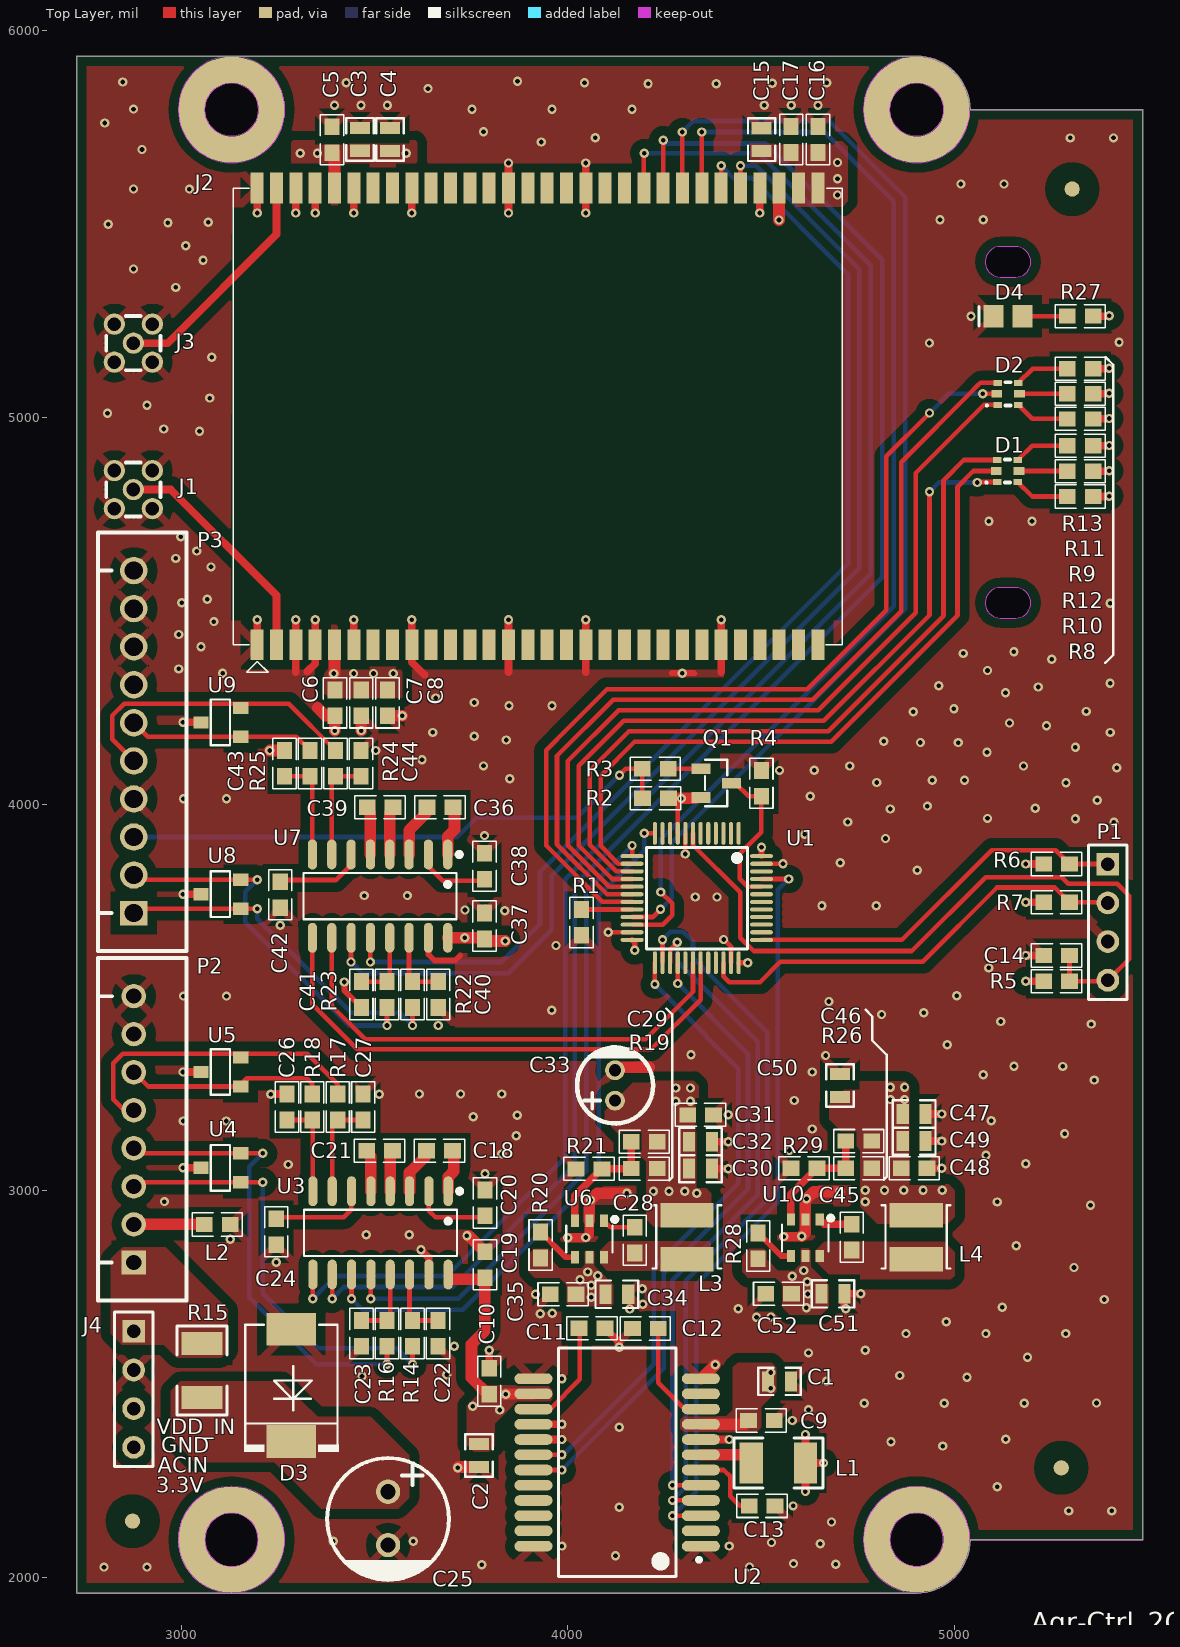
[diagram p0: Top Layer view]
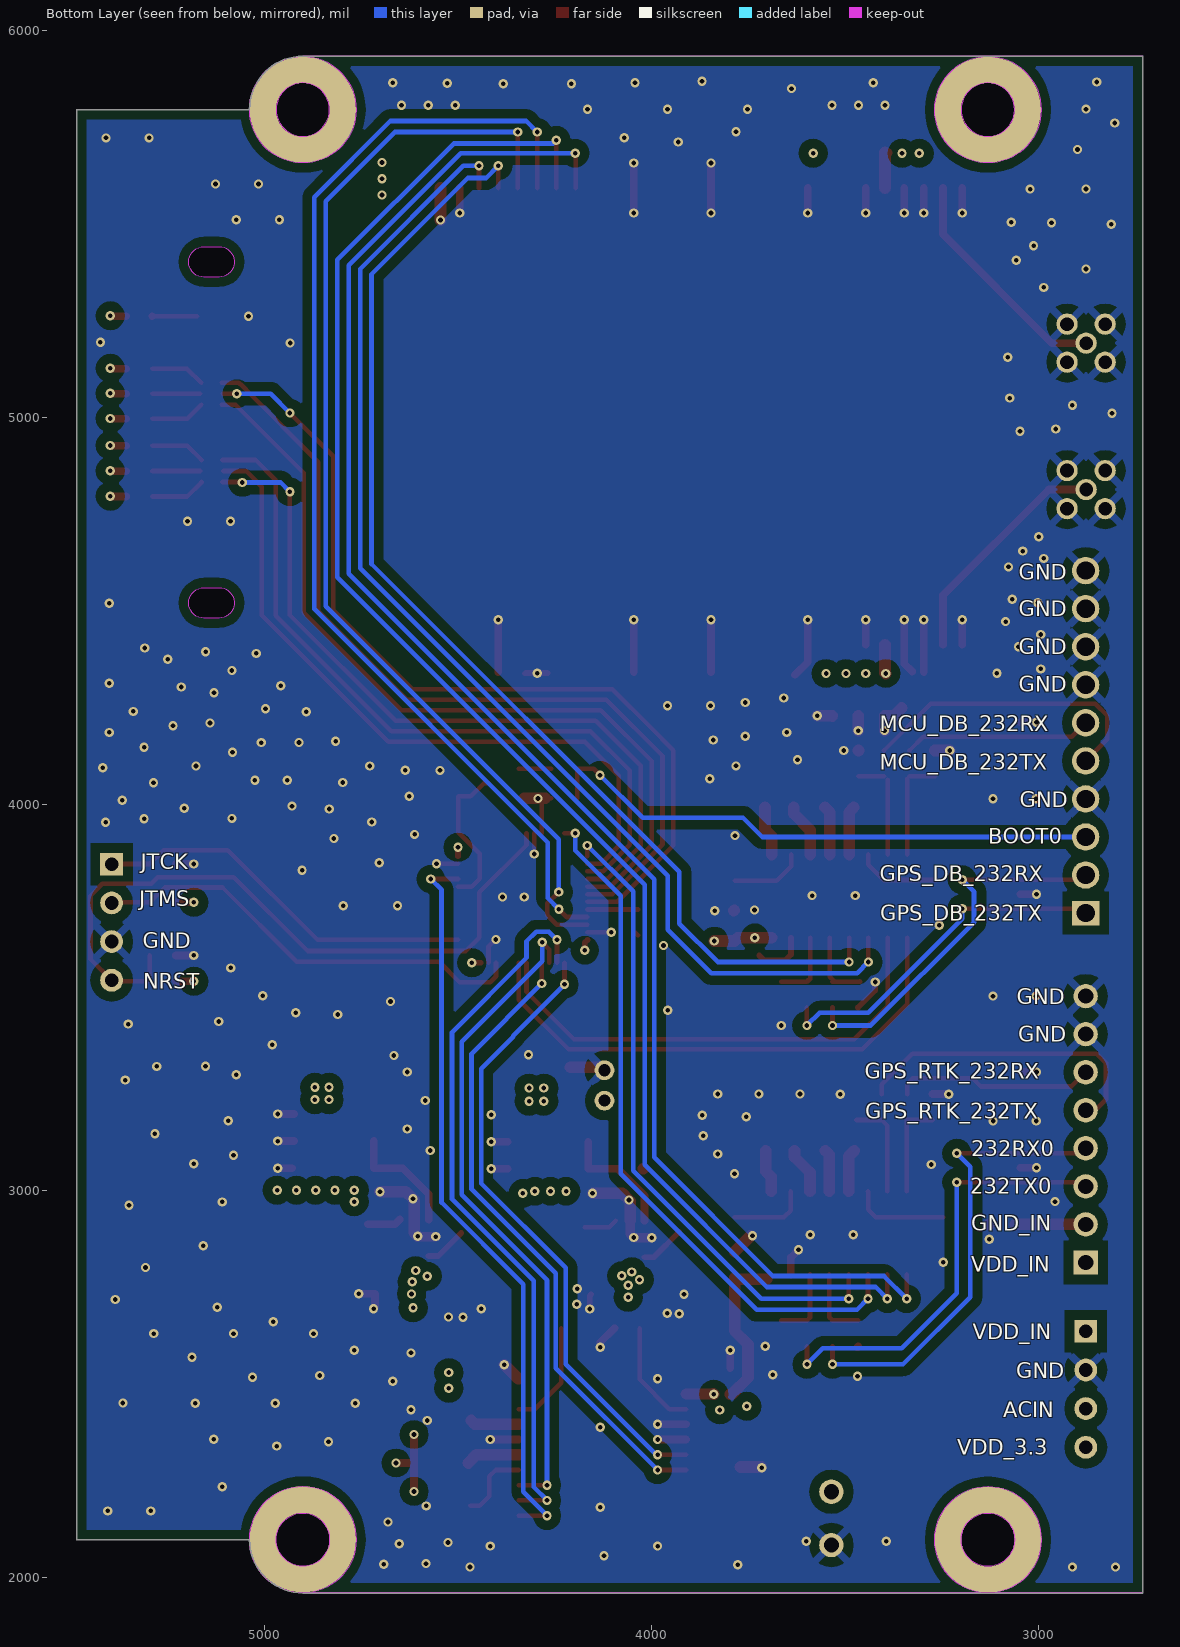
[diagram p1: Bottom Layer view, seen from below]
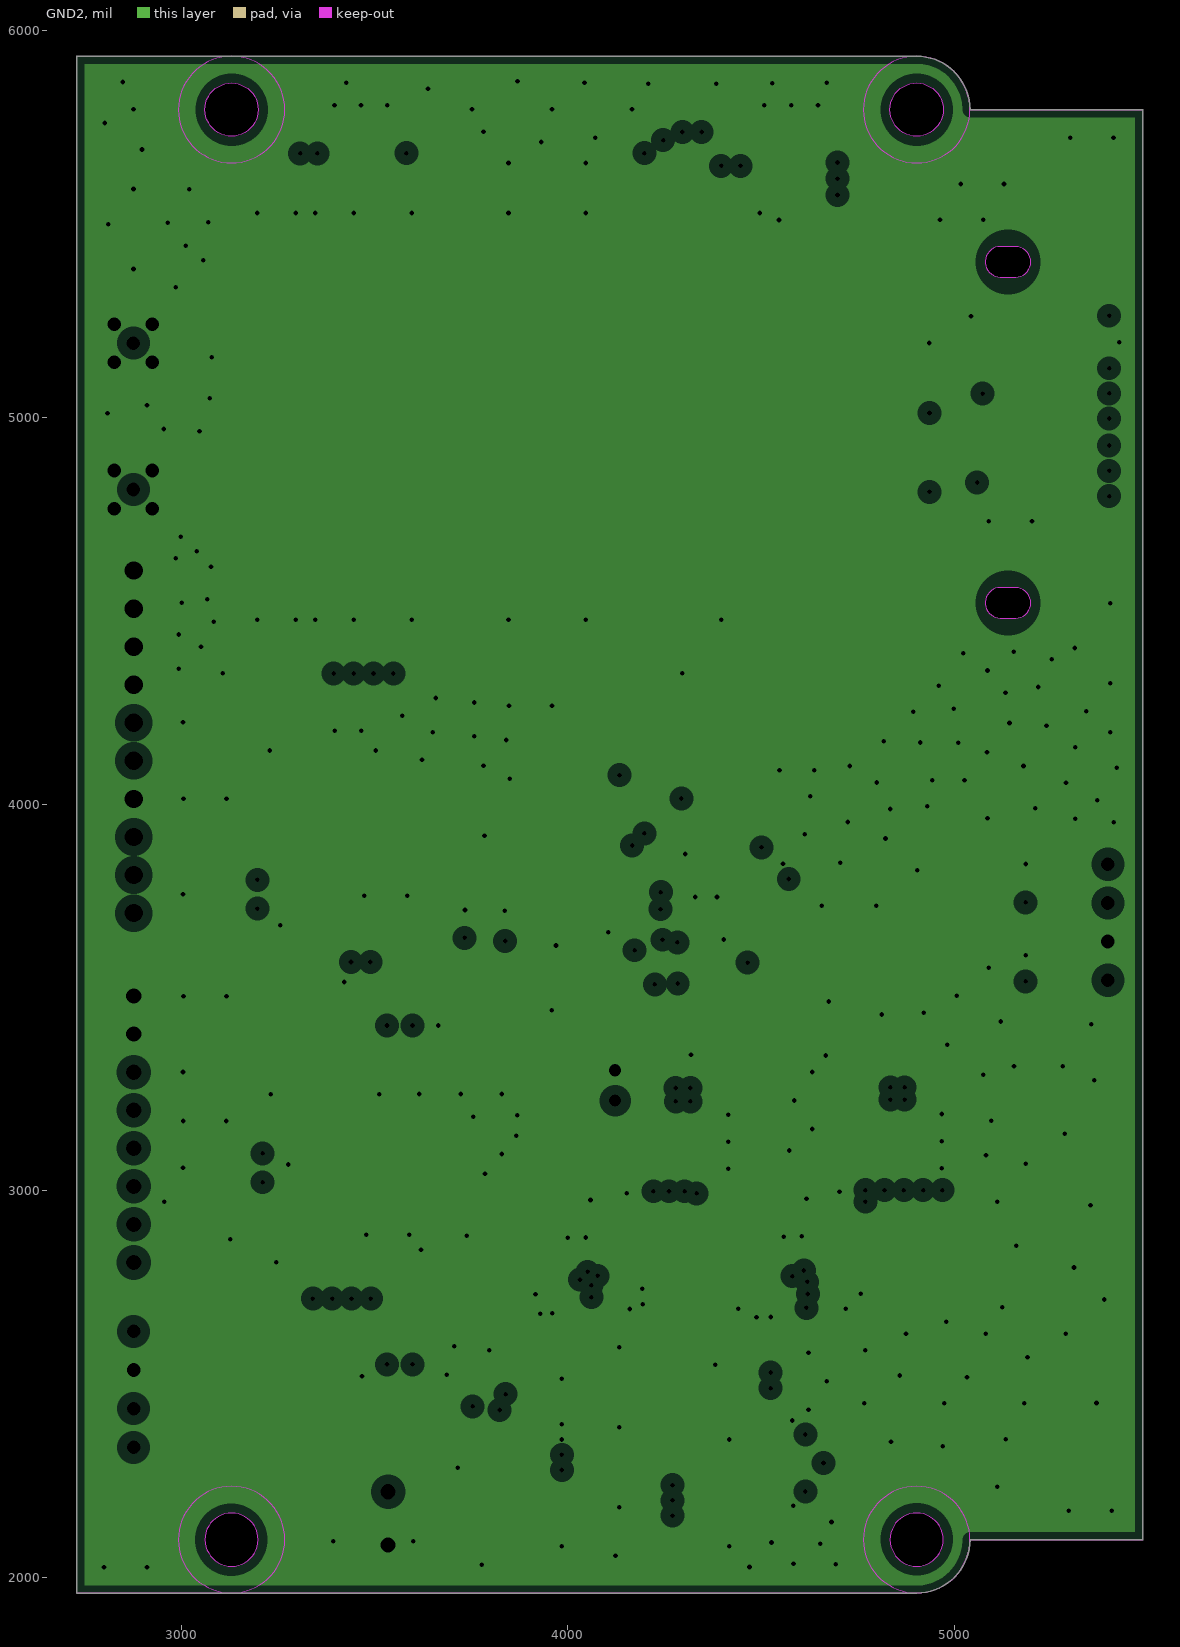
[diagram p2: GND2, clearances drawn from the general rule]
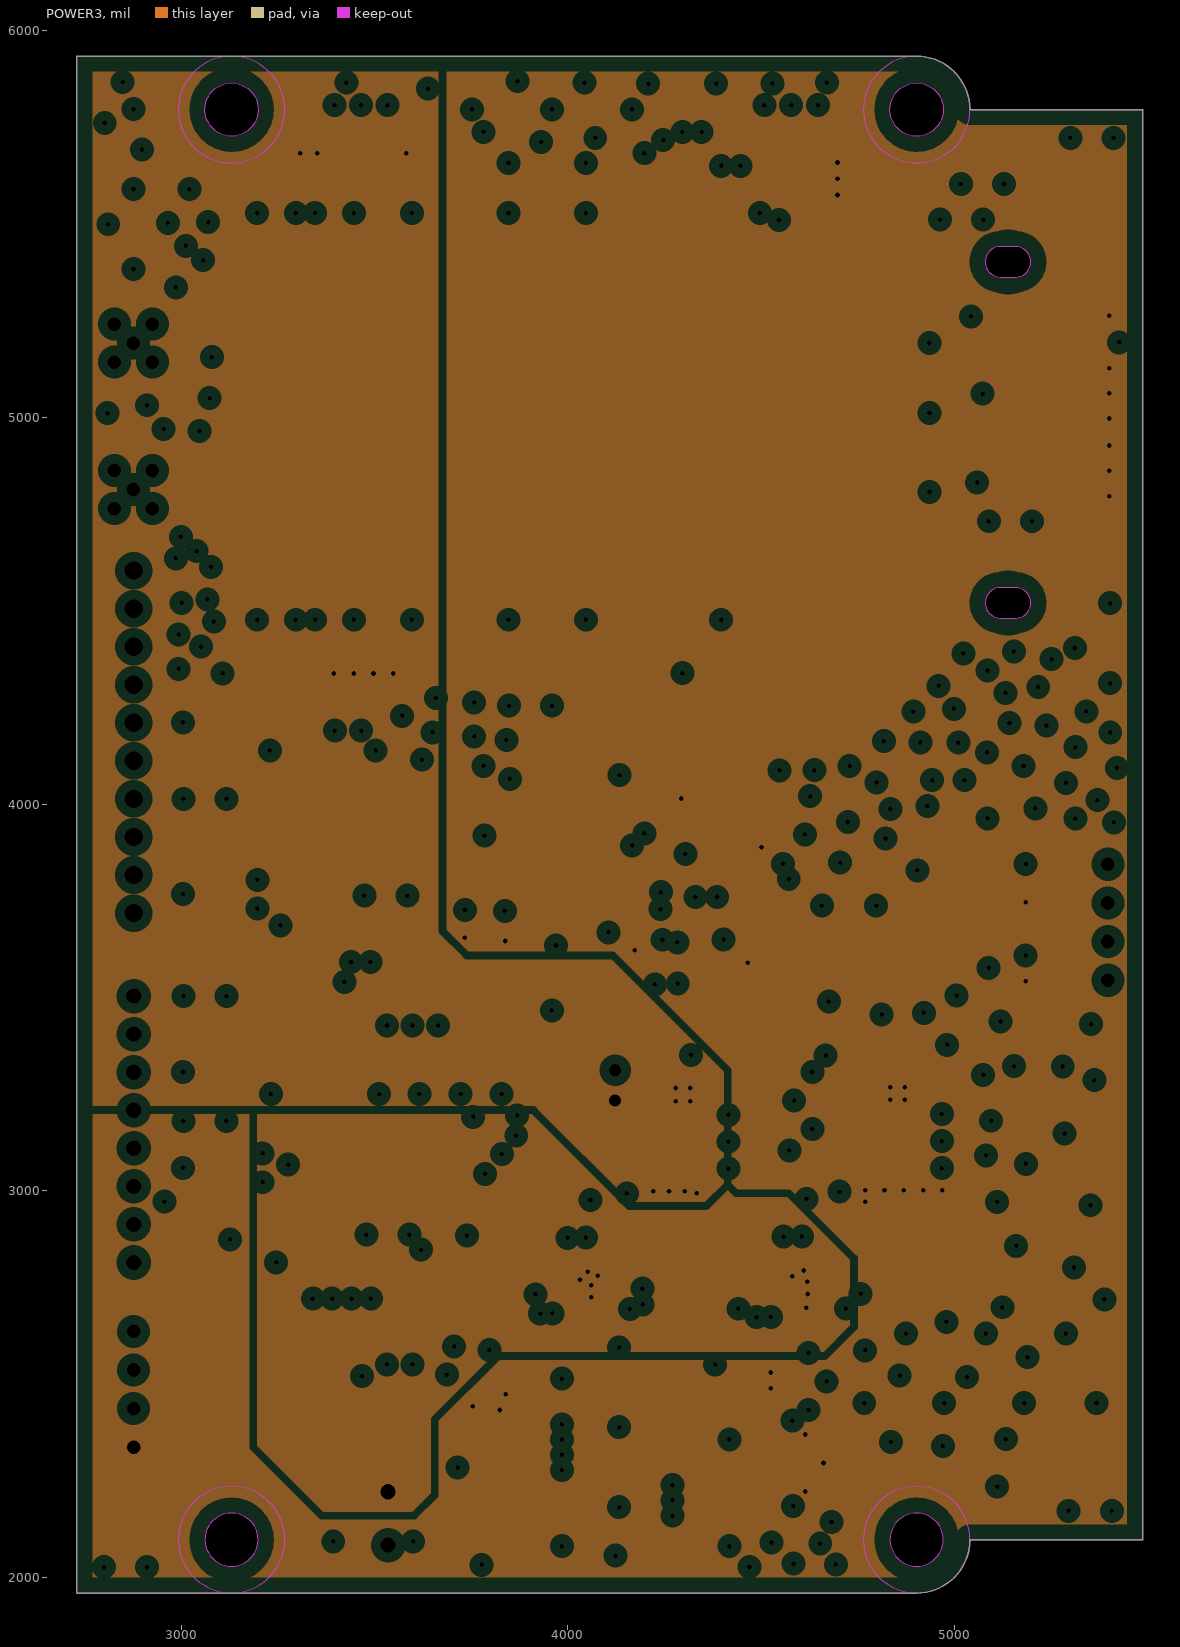
[diagram p3: POWER3, clearances drawn from the general rule]
# Altium PCB MISC84436.PcbDoc (part 1 of 2)
Units mil, origin at the board's own origin, x right, y up, seen from the top; angles counter-clockwise.
Board outline 2756.44 x 3974.35 mil, 4 copper layers (Top Layer, GND2, POWER3, Bottom Layer), stack 23.756 mil thick; 107 components, 89 nets, 422 pads, 390 vias.

## Layer stack, top to bottom
Top Layer: signal copper 1.4
Dielectric: prepreg 2.8, PP-006, Dk 4.1
GND2: plane copper 1.3778, net GND
Dielectric: dielectric 12.6, FR-4, Dk 4.8
POWER3: plane copper 1.3778, net (Multiple Nets)
Dielectric: prepreg 2.8, PP-006, Dk 4.1
Bottom Layer: signal copper 1.4

## Board outline
2730,1959.73 cw(c2730,1960) 2729.74,1960 2729.74,5933.82 cw(c2730,5933.82) 2730,5934.08 4901.63,5934.08 cw(c4901.63,5796.02) 5039.69,5796.29 5485.91,5796.29 cw(c5485.91,5796.02) 5486.17,5796.02 5486.17,2097.8 cw(c5485.91,2097.8) 5485.91,2097.53 5039.69,2097.53 cw(c4901.63,2097.8) 4901.63,1959.73 cw(c4901.63,2097.8) 4901.46,1959.73
cut-out: 3061.08,2097.8 ccw(c3129.97,2097.8) 3129.97,2028.9 ccw(c3129.97,2097.8) 3198.87,2097.8 ccw(c3129.97,2097.8) 3129.97,2166.69 ccw(c3129.97,2097.8)
cut-out: 4832.73,2097.8 ccw(c4901.63,2097.8) 4901.63,2028.9 ccw(c4901.63,2097.8) 4970.52,2097.8 ccw(c4901.63,2097.8) 4901.63,2166.69 ccw(c4901.63,2097.8)
cut-out: 4901.63,5727.12 cw(c4901.63,5796.02) 4832.73,5796.02 cw(c4901.63,5796.02) 4901.63,5864.92 cw(c4901.63,5796.02) 4970.52,5796.02 cw(c4901.63,5796.02)
cut-out: 3129.97,5727.12 cw(c3129.97,5796.02) 3061.08,5796.02 cw(c3129.97,5796.02) 3129.97,5864.92 cw(c3129.97,5796.02) 3198.87,5796.02 cw(c3129.97,5796.02)
cut-out: 5118.15,5362.95 5157.52,5362.95 ccw(c5157.52,5402.32) 5157.52,5441.69 5118.15,5441.69 ccw(c5118.15,5402.32)
cut-out: 5118.15,4481.06 5157.52,4481.06 ccw(c5157.52,4520.43) 5157.52,4559.8 5118.15,4559.8 ccw(c5118.15,4520.43)

## Design rules (kind name [scope] priority, off if disabled: settings)
Clearance mark [HASPAD('FREE-MARK')] p1: gap=50
Clearance GND_Clearance [InNet('GND')] p2: gap=6
Clearance [All] p3: gap=6
ComponentClearance [All] p1: gap=0 collisioncheckmode=3 verticalgap=0 showdistances=FALSE
HoleSize [All] p1: absolutevalues=TRUE maxlimit=500 minlimit=12 maxpercent=80.000 minpercent=20.000
HoleToHoleClearance [All] p1: gap=0 allowstackedmicrovias=TRUE
MinimumSolderMaskSliver [All] p1: minsoldermaskwidth=0
PlaneClearance [All] p1: clearance=25
PlaneConnect [All] p1: planeconnectstyle=Direct reliefexpansion=15 reliefentries=4 reliefconductorwidth=15 reliefairgap=15
PolygonConnect PolygonConnect_1 [ISVIA] p1: connectstyle=Direct reliefconductorwidth=10 reliefentries=4 polygonreliefangle="90 Angle"
PolygonConnect PolygonGND [InNet('GND')] p2: connectstyle=Relief reliefconductorwidth=20 reliefentries=4 polygonreliefangle="45 Angle"
PolygonConnect [All] p3: connectstyle=Direct reliefconductorwidth=10 reliefentries=4 polygonreliefangle="90 Angle"
RoutingVias [All] p1: holewidth=12 width=24 viastyle="Through Hole" minholewidth=12 minwidth=24 maxholewidth=12 maxwidth=24
SilkToSilkClearance [All] p1: silktosilkclearance=0
SilkscreenOverComponentPads SilkToSolderMaskClearance [IsPad] p1: minsilkscreentomaskgap=0
SolderMaskExpansion [All] p1: expansion=2.5
Width [All] p1: maxlimit=30 minlimit=6 preferedwidth=10
20 further rules are at their usual default settings.

## Components (designator, comment, footprint, x,y, rotation, side; value= is the part's Value field where it differs from the comment)
C1 "22uF/10V" C0805 4546.85,2507.09 r0 top
C2 "22uF/10V" C0805 3770.08,2315.3 r270 top
C3 "10uF/25V" C0805 3462.2,5719.29 r270 top
C4 "10uF/25V" C0805 3539.76,5718.9 r270 top
C5 "100nF/50V" 0603 3389.76,5718.11 r90 top
C6 "100pF/50V" 0603 3397.24,4261.81 r270 top
C7 "100pF/50V" 0603 3465.18,4261.81 r90 top
C8 "100nF/50V" 0603 3533.12,4261.81 r90 top
C9 "1uF/25V" 0603 4500,2405.91 r0 top
C10 "100nF/50V" 0603 3796.46,2507.48 r90 top
C11 "1uF/25V" 0603 4062.2,2644.49 r0 top
C12 "1uF/25V" 0603 4200,2643.7 r180 top
C13 "470nF/50V" 0603 4501.97,2185.04 r0 top
C14 "100nF/50V" 0603 5263.63,3608.66 r0 top
C15 "10uF/25V" C0805 4500.79,5718.5 r270 top
C16 "100pF/50V" 0603 4646.46,5718.9 r270 top
C17 "100nF/50V" 0603 4577.05,5718.9 r270 top
C18 "100nF/50V" 0603 3667.56,3103.66 r0 top
C19 "100nF/50V" 0603 3785.16,2808.56 r90 top
C20 "100nF/50V" 0603 3785.16,2968.56 r90 top
C21 "100nF/50V" 0603 3512.76,3103.66 r0 top
C22 "15pF/50V" 0603 3663.78,2631.14 r90 top
C23 "15pF/50V" 0603 3465.75,2631.14 r90 top
C24 "100nF/50V" 0603 3245.32,2894.13 r270 top
C25 "470uF/25V" CAP-TH_BD8.0-P3.50-D1.0-FD 3534.65,2152.76 r270 top
C26 "15pF/50V" 0603 3273.23,3216.54 r90 top
C27 "15pF/50V" 0603 3470.08,3216.54 r90 top
C28 "100nF/50V" 0603 4172.83,2872.28 r90 top
C29 "100pF/50V" 0603 4197.17,3126.8 r180 top
C30 "22uF/10V" C0805 4342.83,3057.28 r0 top
C31 "100nF/50V" 0603 4342.83,3196.31 r0 top
C32 "22uF/10V" C0805 4342.83,3126.8 r0 top
C33 "100uF/10V" CAP-TH_BD5.0-P2.00-D0.8-FD 4121.65,3272.44 r90 top
C34 "10uF/25V" C0805 4126.3,2732.28 r180 top
C35 "100nF/50V" 0603 3987.4,2732.28 r0 top
C36 "100nF/50V" 0603 3668.98,3991.83 r0 top
C37 "100nF/50V" 0603 3783.98,3684.63 r90 top
C38 "100nF/50V" 0603 3783.98,3839.43 r90 top
C39 "100nF/50V" 0603 3513.98,3991.83 r0 top
C40 "15pF/50V" 0603 3664.17,3507.48 r90 top
C41 "15pF/50V" 0603 3465.73,3507.48 r90 top
C42 "100nF/50V" 0603 3255.91,3765.75 r270 top
C43 "15pF/50V" 0603 3266.93,4105.24 r90 top
C44 "15pF/50V" 0603 3464.57,4105.24 r90 top
C45 "100nF/50V" 0603 4733.7,2880 r90 top
C46 "100pF/50V" 0603 4751.97,3128.46 r180 top
C47 "22uF/10V" C0805 4895.24,3198.46 r0 top
C48 "100nF/50V" 0603 4895.24,3058.46 r0 top
C49 "22uF/10V" C0805 4895.24,3128.46 r0 top
C50 "22uF/10V" C0805 4703.54,3272.44 r90 top
C51 "10uF/25V" C0805 4685.2,2733.46 r180 top
C52 "100nF/50V" 0603 4544.76,2733.46 r0 top
D1 "Full-color RGB LED" RGB 5137.01,4861.42 r180 top
D2 "Full-color RGB LED" RGB 5138.19,5061.02 r180 top
D3 "SMCJ18A" SMC_L6.9-W5.9-LS7.9-RD 3284.65,2496.85 r90 top
D4 "RED" LED_0805 5137.8,5261.81 r180 top
J1 "MMCX-KE RF connector" MMCX-TH_ZC11.801KK 2875.98,4813.39 r180 top
J2 "UM482/K823" UM482/K823 3921.06,5002.76 r90 top locked
J3 "MMCX-KE RF connector" MMCX-TH_ZC11.801KK 2875.98,5192.13 r0 top
J4 "Header" HDR1X4 2876.77,2636.61 r270 top
L1 "47uH±20%" 1210 4544.02,2296.06 r180 top
L2 "120Ω ±25% @100MHz" 0603 3092.91,2912.6 r0 top
L3 "2.2uH/2A" IND-SMD_L4.0-W4.0 4307.48,2879.92 r90 top
L4 "2.2uH/2A" IND-SMD_L4.0-W4.0 4900.39,2879.92 r90 top
P1 "Header" HDR1X4 5396.06,3844.49 r270 top locked
P2 "XH-8A" CONN-TH_XH-8A 2877.16,3159.06 r90 top locked
P3 "XH-10A" CONN-TH_10P-P2.50_XH-10A 2877.17,4161.03 r90 top locked
Q1 "8550" SOT-23-SS8550 4383.07,4054.33 r180 top
R1 "10K" 0603 4035.04,3694.09 r90 top
R2 "10K" 0603 4226.14,4015.12 r0 top
R3 "10K" 0603 4225.75,4091.5 r180 top
R4 "10K" 0603 4500.16,4053.7 r270 top
R5 "10K" 0603 5263.63,3541.73 r180 top
R6 "10K" 0603 5263.63,3845.28 r180 top
R7 "10K" 0603 5263.63,3746.06 r180 top
R8 "1.5K" 0603 5324.8,4795.47 r180 top
R9 "1.5K" 0603 5324.8,4996.26 r180 top
R10 "680R" 0603 5324.8,4861.02 r180 top
R11 "680R" 0603 5324.8,5061.22 r180 top
R12 "1K" 0603 5324.8,4926.57 r180 top
R13 "1K" 0603 5324.8,5126.18 r180 top
R14 "4.7Ω,±1%" 0603 3597.77,2631.14 r90 top
R15 "12V/2A" 1210 3053.54,2535.43 r90 top
R16 "4.7Ω,±1%" 0603 3531.76,2631.14 r90 top
R17 "4.7Ω,±1%" 0603 3404.46,3216.54 r270 top
R18 "4.7Ω,±1%" 0603 3338.85,3216.54 r270 top
R19 "75K 1%" 0603 4197.17,3057.28 r0 top
R20 "100K" 0603 3929.13,2859.84 r270 top
R21 "10K" 0603 4054.25,3056.65 r0 top
R22 "4.7Ω,±1%" 0603 3598.02,3507.48 r90 top
R23 "4.7Ω,±1%" 0603 3531.88,3507.48 r90 top
R24 "4.7Ω,±1%" 0603 3398.69,4105.24 r270 top
R25 "4.7Ω,±1%" 0603 3332.81,4105.24 r270 top
R26 "100K" 0603 4751.97,3058.46 r0 top
R27 "1K" 0603 5324.8,5262.01 r0 top
R28 "100K" 0603 4491.73,2857.48 r270 top
R29 "22.1K" 0603 4610.24,3058.46 r0 top
U1 "STM32F103C8T6/GD32F103C8T6" LQFP-48_L7.0-W7.0-P0.50-LS9.0-BL 4333.08,3757.09 r180 top locked
U2 "SCC2130" SCC2130D 4127.15,2297.63 r180 top
U3 "SP3232EEN" SOP16-6.6 3515.16,2891.16 r270 top
U4 "PESD15VL2BT" SOT-23 3102.24,3059.45 r90 top
U5 "PESD15VL2BT" SOT-23 3102.24,3307.09 r90 top
U6 "SY8113B" TSOT-23-6_L2.9-W1.6-P0.95-LS2.8-BR 4055.19,2875.32 r90 top
U7 "SP3232EEN" SOP16-6.6 3513.98,3762.03 r270 top
U8 "PESD15VL2BT" SOT-23 3102.24,3766.93 r90 top
U9 "PESD15VL2BT" SOT-23 3102.24,4211.42 r90 top
U10 "SY8113B" TSOT-23-6_L2.9-W1.6-P0.95-LS2.8-BR 4613.7,2878.46 r90 top

## Footprints (in the part's own frame and the unit in brackets; to place one, negate y for a bottom-side part, rotate by r counter-clockwise, add the part's x,y. Pads: shape width x height; smd on the part's side, far side on the other; paste and mask are expansions set on the pad)
0603 [mm] "贴片带丝印"
  rect 1.1x1 smd: 1(-0.85,0) 2(0.85,0)
  silkscreen extent -1.65,-0.76 1.65,0.76, body extent -1.14,-0.38 1.14,0.38, height 1
1210 [mil] "贴片元件"
  rect 60x106.3 smd: 1(-70,0) 2(70,0)
  silkscreen extent -115,-65 115,65, body extent -65,-50 65,50, height 39
C0805 [mm] "C0805"
  rect 0.8x1.3 smd: 1(-0.75,0) 2(0.75,0)
  silkscreen extent -1.4,-0.9 1.4,0.9
CAP-TH_BD5.0-P2.00-D0.8-FD [mm]
  round 1.3 hole 0.8: 1(-1,0) 2(1,0)
  silkscreen extent -2.5,-2.5 2.5,2.5
CAP-TH_BD8.0-P3.50-D1.0-FD [mm]
  round 1.6 hole 1: 1(-1.75,0) 2(1.75,0)
  silkscreen extent -3.96,-4 4.04,4
CONN-TH_10P-P2.50_XH-10A [mm]
  rect 1.6x1.8 hole 1.2: 1(-11.25,0)
  round 1.8 hole 1.2: 2(-8.75,0) 3(-6.25,0) 4(-3.75,0) 5(-1.25,0) 6(1.25,0) 7(3.75,0) 8(6.25,0) 9(8.75,0) 10(11.25,0)
  silkscreen extent -13.75,-3.45 13.75,2.35
CONN-TH_XH-8A [mm]
  rect 1.6x1.6 hole 1: 1(-8.75,0)
  round 1.6 hole 1: 2(-6.25,0) 3(-3.75,0) 4(-1.25,0) 5(1.25,0) 6(3.75,0) 7(6.25,0) 8(8.75,0)
  silkscreen extent -11.25,-3.46 11.25,2.35
HDR1X4 [mm] "Connector; Header; 4 Position"
  rect 1.5x1.5 hole 0.9: 1(0,0)
  round 1.5 hole 0.9: 2(2.54,0) 3(5.08,0) 4(7.62,0)
  silkscreen extent -1.27,-1.27 8.89,1.27
IND-SMD_L4.0-W4.0 [mm]
  rect 1.6x3.5 smd: 1(-1.45,0) 2(1.45,0)
  silkscreen extent -2.05,-2.25 2.1,2.25
LED_0805 [mm] "贴片二极管"
  rect 1.3x1.5 smd: 1(-0.95,0) 2(0.95,0)
  silkscreen extent 1.91,-0.63 1.91,0.64
LQFP-48_L7.0-W7.0-P0.50-LS9.0-BL [mm]
  oval 0.27x1.5 smd: 1(-2.75,-4.25) 2(-2.25,-4.25) 3(-1.75,-4.25) 4(-1.25,-4.25) 5(-0.75,-4.25) 6(-0.25,-4.25) 7(0.25,-4.25) 8(0.75,-4.25) 9(1.25,-4.25) 10(1.75,-4.25) 11(2.25,-4.25) 12(2.75,-4.25) 25(2.75,4.25) 26(2.25,4.25) 27(1.75,4.25) 28(1.25,4.25) 29(0.75,4.25) 30(0.25,4.25) 31(-0.25,4.25) 32(-0.75,4.25) 33(-1.25,4.25) 34(-1.75,4.25) 35(-2.25,4.25) 36(-2.75,4.25)
  oval 1.5x0.27 smd: 13(4.25,-2.75) 14(4.25,-2.25) 15(4.25,-1.75) 16(4.25,-1.25) 17(4.25,-0.75) 18(4.25,-0.25) 19(4.25,0.25) 20(4.25,0.75) 21(4.25,1.25) 22(4.25,1.75) 23(4.25,2.25) 24(4.25,2.75) 37(-4.25,2.75) 38(-4.25,2.25) 39(-4.25,1.75) 40(-4.25,1.25) 41(-4.25,0.75) 42(-4.25,0.25) 43(-4.25,-0.25) 44(-4.25,-0.75) 45(-4.25,-1.25) 46(-4.25,-1.75) 47(-4.25,-2.25) 48(-4.25,-2.75)
  silkscreen extent -3.33,-3.31 3.3,3.34
MMCX-TH_ZC11.801KK [mm]
  round 1.4 hole 0.9: 1(0,0) 2(-1.25,1.25) 3(1.25,1.25) 4(1.25,-1.25) 5(-1.25,-1.25)
  silkscreen extent -1.78,-1.78 1.78,1.78
RGB [mm]
  rect 0.55x0.4 smd: 1(0.675,0.725) 2(-0.675,0.725) 5(0.675,-0.725) 6(-0.675,-0.725)
  rect 0.7x0.5 smd: 3(0.75,0) 4(-0.75,0)
  silkscreen extent -0.17,-0.76 1.46,0.82
SCC2130D [mm] "SOP, 24-Leads, Body 15.00x8.50mm, Pitch 1.00mm, IPC Medium Density"
  oval 2.5x0.7 smd: 1(-5.5,5.5) 2(-5.5,4.5) 3(-5.5,3.5) 4(-5.5,2.5) 5(-5.5,1.5) 6(-5.5,0.5) 7(-5.5,-0.5) 8(-5.5,-1.5) 9(-5.5,-2.5) 10(-5.5,-3.5) 11(-5.5,-4.5) 12(-5.5,-5.5) 13(5.5,-5.5) 14(5.5,-4.5) 15(5.5,-3.5) 16(5.5,-2.5) 17(5.5,-1.5) 18(5.5,-0.5) 19(5.5,0.5) 20(5.5,1.5) 21(5.5,2.5) 22(5.5,3.5) 23(5.5,4.5) 24(5.5,5.5)
  silkscreen extent -5.5,-7.5 3.85,7.5, body extent -4.25,-7.5 4.25,7.5, height 4.2
SMC_L6.9-W5.9-LS7.9-RD [mm]
  rect 2.158x3.24 smd: 1(3.686,0) 2(-3.686,0)
  silkscreen extent -4.36,-3.1 3.98,3.1
SOP16-6.6 [mil]
  oval 77.6x23.7 smd: 1(-107.7,175) 2(-107.7,125) 3(-107.7,75) 4(-107.7,25) 5(-107.7,-25) 6(-107.7,-75) 7(-107.7,-125) 8(-107.7,-175) 9(107.7,-175) 10(107.7,-125) 11(107.7,-75) 12(107.7,-25) 13(107.7,25) 14(107.7,75) 15(107.7,125) 16(107.7,175)
  silkscreen extent -114,-198 60,211
SOT-23 [mm] "SOT-23"
  rect 0.8x1 smd: 1(-0.95,-1.3) 2(0.95,-1.3) 3(0,1.3)
  silkscreen extent -1.5,-0.61 1.5,0.66
SOT-23-SS8550 [mm]
  rect 1.25x0.7 smd: 1(1,-0.95) 2(1,0.95) 3(-1,0)
  silkscreen extent -0.73,-1.53 0.73,1.53
TSOT-23-6_L2.9-W1.6-P0.95-LS2.8-BR [mm]
  rect 0.8x0.532 smd: 1(1.2,-0.95) 2(1.2,0) 3(1.2,0.95) 4(-1.2,0.95) 5(-1.2,0) 6(-1.2,-0.95)
  silkscreen extent -0.88,-1.82 1.44,1.53
UM482/K823 [mm]
  rect 2.01x0.85 smd: 1(-15,18.415) 2(-15,17.145) 3(-15,15.875) 4(-15,14.605) 5(-15,13.335) 6(-15,12.065) 7(-15,10.795) 8(-15,9.525) 9(-15,8.255) 10(-15,6.985) 11(-15,5.715) 12(-15,4.445) 13(-15,3.175) 14(-15,1.905) 15(-15,0.635) 16(-15,-0.635) 17(-15,-1.905) 18(-15,-3.175) 19(-15,-4.445) 20(-15,-5.715) 21(-15,-6.985) 22(-15,-8.255) 23(-15,-9.525) 24(-15,-10.795) 25(-15,-12.065) 26(-15,-13.335) 27(-15,-14.605) 28(-15,-15.875) 29(-15,-17.145) 30(-15,-18.415) 31(15,-18.415) 32(15,-17.145) 33(15,-15.875) 34(15,-14.605) 35(15,-13.335) 36(15,-12.065) 37(15,-10.795) 38(15,-9.525) 39(15,-8.255) 40(15,-6.985) 41(15,-5.715) 42(15,-4.445) 43(15,-3.175) 44(15,-1.905) 45(15,-0.635) 46(15,0.635) 47(15,1.905) 48(15,3.175) 49(15,4.445) 50(15,5.715) 51(15,6.985) 52(15,8.255) 53(15,9.525) 54(15,10.795) 55(15,12.065) 56(15,13.335) 57(15,14.605) 58(15,15.875) 59(15,17.145) 60(15,18.415)
  silkscreen extent -16.81,-20 15,20

## Part data
C1 C2 C30 C32: library part Cap, "SMD ceramic capacitor,X5R"
C3 C4 C9 C10 C11 C12 C13 C15: library part Cap, "SMD ceramic capacitor,X7R"
C5 C6 C7 C8 C16 C17 C28 C29 C31 C35: library part Cap, "SMD ceramic capacitor"
C14 C45 C46 C47 C48 C49 C51 C52: library part Cap, "Capacitor"
C18 C19 C20 C21 C22 C23 C24 C26 C27 C36 C37 C38 C39 C40 C41 C42 C43 C44: library part Cap, "SMD capacitor,X7R"
C25: library part Cap, "470μF,25V,Ф8×11.5mm,RoHS"
C33: library part Cap2, "100μF,10V,Ф5×7mm,RoHS"
C34: library part Cap, "SMD ceramic capacitor,MLCC"
C50: library part Cap2, "Capacitor"
D1 D2: library part LED1_3, "19-337C/RSBHGHC-M03/2T,EVERLIGHT (Taiwan)"
D3: library part Diode, "TVS diode"
D4: library part LED1, "Red high-brightness LED"
J1 J3: library part CIRCLE
J2: library part UM482, "High-precision GNSS receiver"
J4: library part 2.54, "Single-row straight header,4P,2.54mm"
L1: library part Inductor, "SMD inductor"
L2: library part Inductor, "Ferrite bead"
L3 L4: library part Inductor, "SMD power inductor,cjiang,FNR4026S2R2MT"
P1: library part "Header 4", "Single-row straight header,4P,2.54mm"
P2: library part "Header 8", "8P,pitch 2.5mm,through-hole,BOOMELE"
P3: library part "Header 10", "10P,pitch 2.5mm,through-hole,BOOMELE"
Q1: library part PNP, "PNP Bipolar Transistor"
R1 R2 R3 R4 R5: library part Res, "SMD resistor"
R6 R7 R8 R9 R10 R11 R12 R13 R19 R20 R21 R26 R27 R28 R29: library part Res1, "SMD resistor"
R14 R16 R17 R18 R22 R23 R24 R25: library part RES, "SMD resistor"
R15: library part RES, "Resettable fuse"
U1: library part STM32F103C8T6, "STM32 ARM-based 32-bit MCU with ST/GD GigaDevice"
U2: "MEMS digital gyroscope"
U3 U7: library part SP202ECT
U4 U5 U8 U9: library part PESD12VL2BT

## Free pads (board coordinates)
  round 40 hole 78.74 slot 118.11 at 0 deg unplated: 0(5137.8,4520.47) 0(5137.8,5402.36)
  round 275.59 hole 137.8 unplated: 1(3129.53,2097.64) 1(3130.31,5795.67) 1(4901.57,2098.43) 1(4901.57,5796.06)
  round 39.37 smd mask+59.06: MARK(2874.02,2145.67) MARK(5275.59,2283.46) MARK(5303.94,5590.55)

## Via types
v1: diameter 24, hole 12, Top Layer to Bottom Layer, tented both sides, 252 vias
v2: diameter 24, hole 12, Top Layer to Bottom Layer, 138 vias

## Nets (pads, with @x,y where several pads share a name; then routed paths per layer and width w, separated by ;. In a path a pad name is that pad's centre, name@x,y a point inside that pad or via, vN(x,y) a via of type N, cw(c..) or ccw(c..) an arc to the next point about the centre after c; other vN are vias at no path point)
232RX0: P2.4 R16.1 U4.2 | length 1199.2
  Top Layer w12: P2.4@2877.17,3109.84 2885.04,3109.84 2898.03,3096.85 U4.2@3153.43,3096.85 v1(3210.24,3096.85) ; v1(3531.76,2551.21) R16.1@3531.76,2597.68
  Bottom Layer w12: v1(3210.24,3096.85) 3175.59,3062.2 3175.59,2725.2 3349.57,2551.21 v1(3531.76,2551.21)
232TX0: P2.3 R14.1 U4.1 | length 1135
  Top Layer w12: P2.3@2877.17,3011.42 2887.8,3022.05 U4.1@3153.43,3022.05 v1(3210.24,3022.05) ; v1(3597.91,2551.21) R14.1@3597.91,2597.68
  Bottom Layer w12: v1(3210.24,3022.05) 3210.24,2734.64 3352.36,2592.52 3556.6,2592.52 v1(3597.91,2551.21)
ACIN: J4.3
BOOT0: P3.3 R2.1 R3.2 | length 1464.8
  Top Layer w12: v1(4133.07,4074.8) 4149.76,4091.5 R3.2@4192.28,4091.5 4192.28,4015.51 R2.1@4192.68,4015.12
  Bottom Layer w12: P3.3@2877.17,3914.96 3713.78,3914.96 3763.39,3964.57 4022.83,3964.57 v1(4133.07,4074.8)
CPU-URX0: U1.31 U7.9 | length 1372.8
  Top Layer w12: U7.9@3338.98,3654.33 3338.98,3481.89 3454.72,3366.14 4214.57,3366.14 4342.91,3494.49 U1.31@4342.91,3589.78
CPU-UTX0: U1.30 U7.10 | length 1272.4
  Top Layer w12: U7.10@3388.98,3654.33 3388.98,3477.95 3475.2,3391.73 4200.39,3391.73 4323.24,3514.58 U1.30@4323.24,3589.78
GND: C1.2 C2.2 C3.1 C4.1 C5.2 C6.2 C7.1 C8.1 C9.2 C10.2 C11.2 C12.2 C13.2 C14.1 C15.1 C16.1 C17.1 C19.2 C20.2 C22.1 C23.1 C24.2 C25.2 C26.2 C27.2 C30.2 C31.2 C32.2 C33.2 C34.1 C35.1 C37.2 C38.2 C40.1 C41.1 C42.2 C43.2 C44.2 C47.2 C48.2 C49.2 C50.2 C51.1 C52.1 D3.1 D4.2 J1.2 J1.3 J1.4 J1.5 J2.1 J2.3 J2.4 J2.6 J2.9 J2.14 J2.18 J2.25 J2.33 J2.34 J2.43 J2.47 J2.52 J2.55 J2.57 J2.58 J2.60 J3.2 J3.3 J3.4 J3.5 J4.2 L2.2 P1.3 P2.7 P2.8 P3.4 P3.7 P3.8 P3.9 P3.10 R1.1 R4.1 R6.2 R21.1 R29.1 U1.8 U1.23 U1.35 U1.47 U2.1 U2.8 U2.12 U2.13 U2.16 U2.17 U2.24 U3.15 U4.3 U5.3 U6.2 U7.15 U8.3 U9.3 U10.2 | length 4279
  Top Layer w12: R1.1@4035.04,3660.63 R1.1@4042.92,3668.52 ; v1(4104.34,3668.52) U1.23@4165.75,3668.52 ; v1(4295.67,4338.58) 4296.85,4337.4 v1@4297.64,4337.4 ; v1@4296.06,4338.98 v1@4297.64,4337.4 ; v1(4303.54,3870.87) U1.8@4303.54,3924.41 ; 4328.35,4337.4 v1@4297.64,4337.4 ; v1(4402.36,3650) 4421.65,3630.71 U1.35@4421.65,3589.78 ; U1.47@4500.4,3845.67 v1@4555.51,3845.67 ; v1(5042.13,5261.42) v1@5042.52,5261.81
  Top Layer w15: v1(3421.65,3539.76) 3421.65,3518.09 C41.1@3465.73,3474.02 ; U7.15@3638.98,3654.33 3638.98,3611.02 3654.72,3595.28 3707.64,3595.28 3721.17,3608.8 ; C34.1@4155.83,2732.28 4159.76,2728.35 v1(4159.76,2694.09) ; 4325.98,4338.19 4325.2,4338.98 v1@4296.06,4338.98 ; v1@4552.76,2881.49 v1(4557.72,2881.49) ; v1@4296.06,4338.98 4268.9,4338.98 4268.5,4338.58 v1(4295.67,4338.58) v1@4296.06,4338.98
  Top Layer w20: v1(3004.33,3059.45) U4.3@3046.06,3059.45 ; v1(3004.33,3307.09) U5.3@3046.06,3307.09 ; v1(3004.33,3766.93) U8.3@3046.06,3766.93 ; v1(3004.33,4211.42) U9.3@3046.06,4211.42 ; J2.1@3196.06,4412.2 v1(3196.06,4476.77) ; v1(3196.06,5528.74) J2.60@3196.06,5593.31 ; v1(3231.5,3250) C26.2@3273.23,3250 ; 3296.06,4341.73 J2.3@3296.06,4412.2 v1(3296.06,4476.77) ; v1(3296.06,5528.74) J2.58@3296.06,5593.31 ; 3325.59,4342.91 3346.06,4363.39 J2.4@3346.06,4412.2 v1(3346.06,4476.77) ; v1(3346.06,5528.74) J2.57@3346.06,5593.31 ; J2.6@3446.06,4412.2 v1(3446.06,4476.77) ; v1(3446.06,5528.74) J2.55@3446.06,5593.31 ; C23.1@3464.96,2597.68 C23.1@3467.32,2595.32 ; v1(3596.06,4476.77) J2.9@3596.06,4412.2 3596.06,4367.32 3628.74,4334.65 ; v1(3596.06,5528.74) J2.52@3596.06,5593.31 ; v1(3619.68,2847.64) 3640.16,2827.17 U3.15@3640.16,2783.46 ; C10.2@3796.46,2540.94 v1(3796.46,2587.64) ; 3846.06,4341.73 J2.14@3846.06,4412.2 v1(3846.06,4476.77) ; v1(3846.06,5528.74) J2.47@3846.06,5593.31 v1(3846.06,5657.87) ; U2.17@3910.61,2356.69 v1(3984.21,2356.69) ; U2.16@3910.61,2396.06 v1(3984.21,2396.06) ; 4046.06,4341.73 J2.18@4046.06,4412.2 v1(4046.06,4476.77) ; v1(4046.06,5528.74) J2.43@4046.06,5593.31 v1(4046.06,5657.87) ; C11.2@4095.67,2644.49 4132.28,2607.87 ; U2.8@4343.69,2356.69 v1(4417.28,2356.69) ; C30.2@4372.36,3057.28 v1(4414.49,3057.28) ; C32.2@4372.36,3126.8 v1(4414.49,3126.8) ; 4396.06,4341.73 J2.25@4396.06,4412.2 v1(4396.06,4476.77) ; v1(4496.06,5528.74) J2.34@4496.06,5593.31 ; v1(4718.66,2695.28) 4714.72,2699.21 C51.1@4714.72,2733.46 v1(4756.85,2733.46) ; C49.2@4924.76,3128.46 v1(4966.89,3128.46) ; C47.2@4924.76,3198.46 v1(4966.89,3198.46) ; C48.2@4928.7,3058.46 v1(4966.89,3058.46) ; v1(5183.46,3608.66) C14.1@5230.16,3608.66 ; v1(5183.46,3845.28) R6.2@5230.16,3845.28
  Top Layer w25: v1(3999.21,2878.35) 4045.28,2878.35 v1(4046.06,2879.13) 4055.19,2888.26 U6.2@4055.19,2922.56 ; v1(4557.72,2881.49) 4603.79,2881.49 v1(4604.57,2882.28)
  Top Layer w30: L2.2@3125.98,2912.99 L2.2@3126.38,2912.6 ; v1(3228.74,4138.7) C43.2@3266.93,4138.7 C43.2@3267.32,4139.09 ; 3352.56,4248.62 3372.83,4228.35 C6.2@3397.24,4228.35 v1(3397.24,4190.16) ; C44.2@3464.17,4138.31 C44.2@3464.57,4138.7 ; C7.1@3464.79,4228.74 C7.1@3465.18,4228.35 v1(3465.18,4190.16) ; C8.1@3532.72,4227.95 C8.1@3533.12,4228.35 v1(3571.31,4228.35) ; v1@3716.49,2285.78 C2.2@3770.08,2285.78 ; v1@3743.33,2883.86 C19.2@3785.16,2842.03 ; C37.2@3785.83,3725.2 C37.2@3787.01,3724.02 ; R21.1@4020.79,3056.65 R21.1@4021.18,3057.05 ; U6.2@4055.19,2922.56 4055.19,2972.91 v1(4058.27,2975.98) 4075.59,2993.31 v1(4152.36,2993.31) ; C33.2@4121.65,3311.81 4129.53,3319.68 4210.24,3319.68 ; U2.12@4343.69,2514.17 4344.48,2514.17 v1(4380.71,2550.39) ; v1(4545.67,5510.63) 4545.67,5592.91 J2.33@4546.06,5593.31 ; v1(4604.57,2882.28) 4613.7,2891.41 U10.2@4613.7,2925.7 4613.7,2976.05 v1(4616.78,2979.13) 4635.29,2997.64 v1(4701.97,2997.64)
  other v1: 2800,2026.77 2911.42,2026.77 3776.77,2032.68 4122.83,2056.3 3984.21,2081.09 4417.28,2081.09 4526.38,2090.55 3392.91,2093.31 3599.68,2093.31 5294.88,2172.05 5406.3,2172.05 4132.28,2181.73 4582.13,2185.04 3714.57,2283.86 4132.28,2388.5 4580.16,2405.91 4622.1,2433.49 4766.14,2450.79 4972.91,2450.79 5179.68,2450.79 4668.8,2507.09 3984.21,2514.17 3467.32,2520.47 3686.61,2524.41 4622.1,2580.68 4132.28,2595.28 3705.51,2597.68 4874.02,2630.71 5080.79,2630.71 5287.56,2630.71 4487.4,2673.23 4524.8,2673.62 3927.95,2682.28 3959.45,2683.07 4440.55,2694.88 4193.31,2706.3 3915.94,2732.09 4192.13,2746.85 3245.32,2815 3126.38,2874.41 3738.58,2883.86 3478.35,2886.61 3589.76,2886.61 2956.3,2972.05 3785.35,3043.96 3276.38,3068.11 3828.74,3095.28 4572.44,3104.33 3866.14,3142.52 4631.73,3159.87 3005.12,3180.32 3116.54,3180.32 3754.72,3191.34 3868.5,3195.28 4414.49,3196.31 4585.03,3233.46 3511.81,3250 3615.75,3250.39 3722.18,3250.39 3828.61,3250.39 5361.02,3286.22 5073.62,3300 4631.73,3307.06 5153.54,3322.2 4666.14,3350 4318.11,3351.57 3664.17,3427.55 3958.27,3466.54 3005.51,3503.54 3116.93,3503.54 3968.9,3634.25 3255.91,3686.61 3836.61,3724.02 3733.46,3725.98 4329.13,3759.84 4385.43,3759.84 3473.23,3763.39 3584.65,3763.39 4555.91,3845.67 3783.98,3918.56 3005.51,4013.78 3116.93,4013.78 4626.38,4020.47 4546.86,4087.17 3502.76,4138.7 3847.24,4254.72 3958.66,4254.72 5401.97,4312.91 5401.97,4519.69 5088.58,4731.5 5200,4731.5 4934.65,5192.52 5425.2,5194.09 2876.38,5383.86 4962.2,5511.42 5073.62,5511.42 2876.38,5590.63 5016.14,5603.54 5127.56,5603.54 5299.21,5722.83 5410.63,5722.83 2876.38,5797.4 3751.81,5796.85 3958.58,5796.85 4165.35,5796.85 3396.06,5807.65 3464.53,5807.65 3532.99,5807.65 4507.65,5807.65 4577.05,5807.65 4646.46,5807.65
  other v2: 4469.29,2027.17 4692.52,2033.86 4583.07,2035.83 4652.36,2087.4 4681.5,2143.31 5109.84,2234.65 4969.29,2339.76 4835.43,2350.79 5132.28,2357.48 5366.93,2451.18 5031.89,2518.11 4857.87,2522.44 5188.19,2569.68 4768.5,2587.4 4978.35,2661.02 5123.23,2698.82 5387.01,2718.9 5308.66,2801.57 5159.06,2857.48 5351.18,2962.6 5109.84,2971.26 5183.86,3069.68 5081.1,3091.73 5284.25,3147.64 5094.49,3181.1 5279.53,3321.65 4980.71,3377.56 5353.15,3431.1 5118.9,3437.8 4811.02,3455.91 4920.08,3460.24 4674.8,3489.37 5005.12,3504.72 5087.8,3576.38 4656.69,3737.4 4796.85,3737.4 4903.54,3828.74 4703.94,3848.43 4821.26,3911.02 4612.6,3921.65 5411.81,3952.76 4723.62,3953.54 5312.2,3962.2 5085.04,3962.99 4833.46,3987.4 5208.66,3988.98 4929.53,3994.88 5368.9,4010.24 5287.8,4055.12 4798.43,4055.91 4941.73,4061.81 5025.59,4061.81 3849.61,4065.35 4637.01,4087.8 5419.29,4093.7 4728.35,4098.43 5177.95,4098.43 3781.5,4098.82 3622.44,4114.96 5083.46,4133.86 5312.2,4147.24 4911.42,4159.45 5009.45,4159.06 4816.93,4162.6 3840.55,4165.75 3757.48,4175.2 3650,4185.43 5402.36,4185.43 5237.4,4202.76 5141.73,4209.84 4892.91,4238.98 5340.55,4239.76 4998.03,4246.46 3757.48,4262.6 3658.27,4274.41 5131.5,4287.8 5216.14,4302.76 4958.66,4305.91 3106.69,4338.19 5085.04,4345.67 2993.31,4349.61 5250.79,4374.8 5022.44,4389.76 5153.15,4394.09 5310.63,4403.54 3050.79,4407.09 2993.31,4438.58 3084.25,4472.05 3000.79,4520.47 3067.32,4529.53 3076.77,4613.39 2985.83,4635.43 3039.76,4654.33 2998.82,4691.34 3046.85,4964.57 2954.33,4970.08 2809.06,5011.02 2911.42,5031.5 3073.23,5050 3078.74,5155.91 2985.83,5336.22 3056.3,5406.69 3011.81,5443.7 2811.02,5499.61 2965.35,5503.15 3069.29,5505.12 3020.87,5590.55 2898.43,5692.91 3930.71,5712.2 4070.47,5723.23 3781.5,5738.58 2801.97,5761.42 3637.8,5850.39 4207.09,5862.99 4383.07,5862.99 4528.35,5864.17 3426.77,5865.75 4042.52,5865.75 4669.29,5865.75 2848.43,5867.32 3869.29,5869.69
GND_IN: L2.1 P2.2 | length 182.4
  Top Layer w30: P2.2@2877.17,2912.99 3059.06,2912.99 L2.1@3059.45,2912.6
GPS_DB_232RX: P3.2 R23.1 U8.2 | length 969.8
  Top Layer w12: P3.2@2877.17,3816.54 2889.37,3804.33 3148.43,3804.33 v1(3196.46,3804.33) ; v1(3531.88,3427.55) R23.1@3531.88,3474.02
  Bottom Layer w12: v1(3196.46,3804.33) 3165.75,3773.62 3165.75,3694.88 3433.08,3427.55 v1(3531.88,3427.55)
GPS_DB_232TX: P3.1 R22.1 U8.1 | length 912.6
  Top Layer w12: P3.1@2877.17,3718.11 2888.58,3729.53 3148.43,3729.53 v1(3196.46,3729.53) ; v1(3598.02,3427.55) R22.1@3598.02,3474.02
  Bottom Layer w12: v1(3196.46,3729.53) 3196.46,3703.14 3439.37,3460.24 3565.34,3460.24 v1(3598.02,3427.55)
GPS_RTK_232RX: P2.6 R18.1 U5.1 | length 518.1
  Top Layer w12: P2.6@2877.17,3306.69 2914.17,3269.69 3148.43,3269.69 3169.69,3290.94 3324.02,3290.94 3338.85,3276.12 R18.1@3338.85,3250
GPS_RTK_232TX: P2.5 R17.1 U5.2 | length 807.1
  Top Layer w12: P2.5@2877.17,3208.27 2852.36,3208.27 2824.41,3236.22 2824.41,3330.31 2848.82,3354.72 3325.59,3354.72 3404.46,3275.85 R17.1@3404.46,3250
GPS_RXD1: J2.36 U7.12 | length 3053.4
  Top Layer w12: v1(3488.98,3591.77) U7.12@3488.98,3654.33 ; J2.36@4396.06,5593.31 v1(4396.06,5650.79)
  Bottom Layer w12: v1(3488.98,3591.77) 3828.78,3591.77 3927.76,3690.75 3927.76,3824.61 4724.02,4620.87 4724.02,5370.47 4475.2,5619.29 4427.56,5619.29 v1(4396.06,5650.79)
GPS_TXD1: J2.35 U7.11 | length 3153.7
  Top Layer w12: v1(3438.98,3591.77) U7.11@3438.98,3654.33 ; J2.35@4446.06,5593.31 v1(4446.06,5650.79)
  Bottom Layer w12: v1(3438.98,3591.77) 3467.76,3562.99 3845.67,3562.99 3958.27,3675.59 3958.27,3814.17 4753.62,4609.53 4753.62,5383.78 4486.61,5650.79 v1(4446.06,5650.79)
JTCK: P1.1 R6.1 U1.37 | length 1007
  Top Layer w12: U1.37@4500.4,3648.82 4863.78,3648.82 5096.06,3881.1 5261.27,3881.1 R6.1@5297.09,3845.28 5395.28,3845.28 P1.1@5396.06,3844.49
JTMS: P1.2 R7.1 U1.34 | length 1153.4
  Top Layer w12: U1.34@4401.98,3589.78 4401.98,3554.72 4417.32,3539.37 4496.46,3539.37 4549.21,3592.13 4917.32,3592.13 5109.45,3784.25 5258.9,3784.25 R7.1@5297.09,3746.06 5394.49,3746.06 P1.2@5396.06,3744.49
LCD1-4_PH4/TXD4: J2.38 U1.21 | length 2999.9
  Top Layer w12: U1.21@4165.75,3707.89 4218.91,3707.89 v1(4239.37,3728.35) ; J2.38@4295.67,5593.31 v1(4295.67,5738.03)
  Bottom Layer w12: v1(4239.37,3728.35) 4268.11,3757.09 4268.11,3900.79 4872.05,4504.72 4872.05,5569.69 4675.2,5766.54 4324.17,5766.54 v1(4295.67,5738.03)
LCD1-5_PH5/RXD4: J2.37 U1.22 | length 2937.5
  Top Layer w12: U1.22@4165.76,3688.2 4245.28,3688.2 4269.29,3712.2 4269.29,3743.31 v1(4240.16,3772.44) ; J2.37@4345.67,5593.31 v1(4345.67,5738.03)
  Bottom Layer w12: v1(4240.16,3772.44) 4240.16,3909.06 4842.44,4511.34 4842.44,5559.13 4663.54,5738.03 v1(4345.67,5738.03)
LCD1-6_PH6/TX5: J2.39 U3.10 | length 4321.8
  Top Layer w12: v1(3390.16,2720.91) U3.10@3390.16,2783.46 ; J2.39@4246.06,5593.31 v2(4246.06,5716.93)
  Bottom Layer w12: v1(3390.16,2720.91) 3420.43,2751.18 3701.97,2751.18 4017.72,3066.93 4017.72,3791.34 4812.83,4586.46 4812.83,5407.24 4511.81,5708.27 4254.72,5708.27 v2(4246.06,5716.93)
LCD1-7_PH7/RX5: J2.40 U3.9 | length 4298.3
  Top Layer w12: v1(3340.16,2720.91) U3.9@3340.16,2783.46 ; J2.40@4196.06,5593.31 4196.06,5682.28 v2(4197.24,5683.46)
  Bottom Layer w12: v1(3340.16,2720.91) 3398.78,2779.53 3686.22,2779.53 3993.31,3086.61 3993.31,3805.91 4783.23,4595.83 4783.23,5393.94 4493.7,5683.46 v2(4197.24,5683.46)
LED1_B: D1.5 U1.15 | length 1922.5
  Top Layer w12: 4056.06,4086.95 4056.06,3894.58 4124.65,3826 U1.15@4165.75,3826 ; 4056.3,4086.95 4157.82,4188.47 4672.72,4188.47 4971.26,4487.01 4971.26,4837.4 5023.82,4889.96 D1.5@5110.43,4889.96